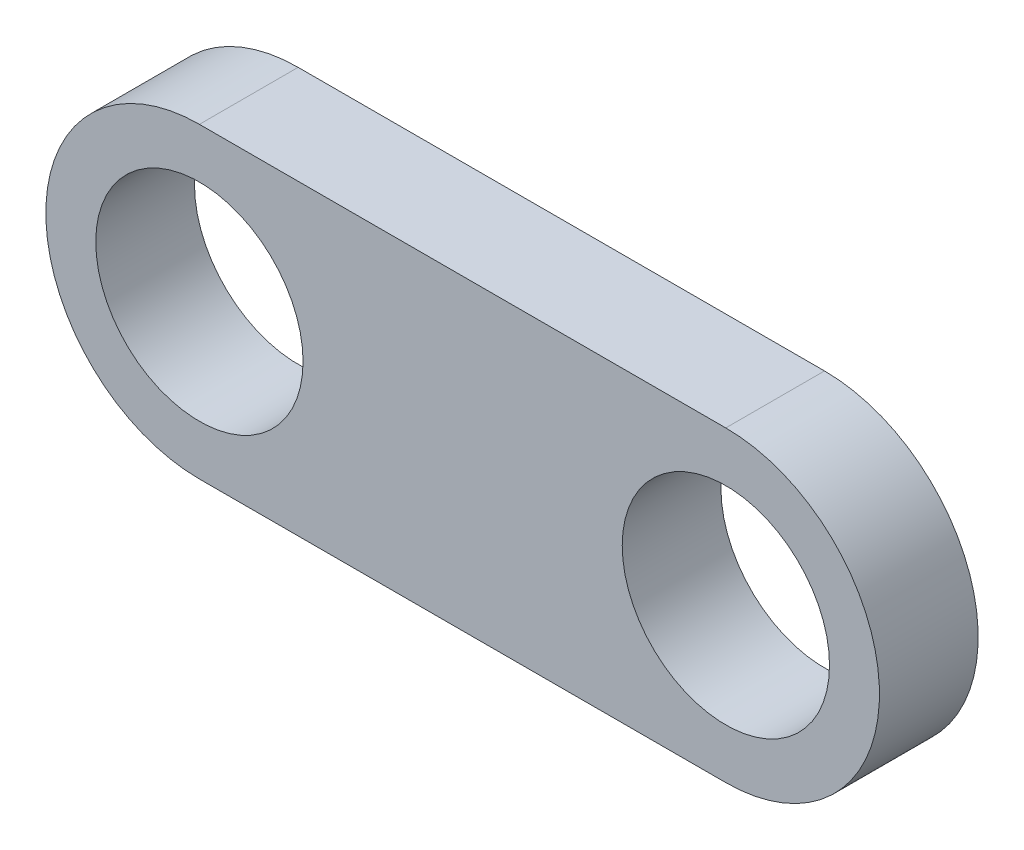
SolidWorks part; units mm, degrees
ref_plane "Front Plane" through (0, 0, 0) normal (0, 0, 1) x (1, 0, 0)
ref_plane "Top Plane" through (0, 0, 0) normal (0, 1, 0) x (1, 0, 0)
ref_plane "Right Plane" through (0, 0, 0) normal (1, 0, 0) x (0, 0, -1)
other "Configuration Table"
sketch "Sketch1" plane through (0, 0, 0) normal (0, 0, 1) x (1, 0, 0)
  line L0 (-0.0017, -0.005) -> (26.1282, 0.0174) construction
  line L1 (7.4641, 5.4527) -> (26.1254, 5.4623)
  line L2 (7.4641, -5.4373) -> (26.1282, -5.4276)
  circle A0 centre (7.4641, 0.0077) radius 3.6746
  circle A1 centre (26.1282, 0.0174) radius 3.6746
  arc A2 (7.4641, 5.4527) -> (7.4697, -5.4373) centre (7.4641, 0.0077) ccw
  arc A4 (26.1282, -5.4276) -> (26.1254, 5.4623) centre (26.1282, 0.0174) ccw
  arc A5 (10.6046, 5.4543) -> (10.6192, -5.4356) centre (-0.0017, -0.005) ccw construction
  arc A9 (11.2821, -3.8744) -> (11.9271, 0.0052) centre (-0.0017, -0.005) ccw construction
extrude "Boss-Extrude1" add sketch "Sketch1" along normal up to surface (3.5 mm away) contours L2 A4 L1 A2 A0 A1
